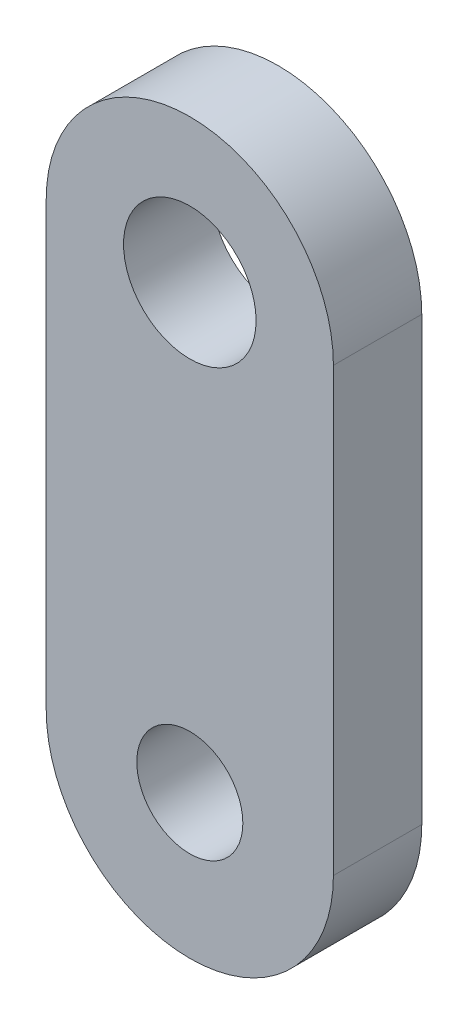
SolidWorks part; units mm, degrees
material "Plain Carbon Steel"
ref_plane "Front Plane" through (0, 0, 0) normal (0, 0, 1) x (1, 0, 0)
ref_plane "Top Plane" through (0, 0, 0) normal (0, 1, 0) x (1, 0, 0)
ref_plane "Right Plane" through (0, 0, 0) normal (1, 0, 0) x (0, 0, -1)
sketch "Sketch1" plane through (0, 0, 0) normal (0, 0, 1) x (1, 0, 0)
  line L0 (0, -1949.1539) -> (0, 95508.5399) construction
  line L1 (6.5, 0) -> (6.5, -20)
  line L2 (-6.5, -20) -> (-6.5, 0)
  circle A0 centre (0, 0) radius 3
  circle A1 centre (0, -20) radius 2.4
  arc A2 (6.5, 0) -> (-6.5, 0) centre (0, 0) ccw
  arc A3 (-6.5, -20) -> (6.5, -20) centre (0, -20) ccw
  dimension "D1" = 6.5
  dimension "D2" = 6
  dimension "D3" = 4.8
  dimension "D4" = 20
extrude "Boss-Extrude1" add sketch "Sketch1" along normal blind 4
